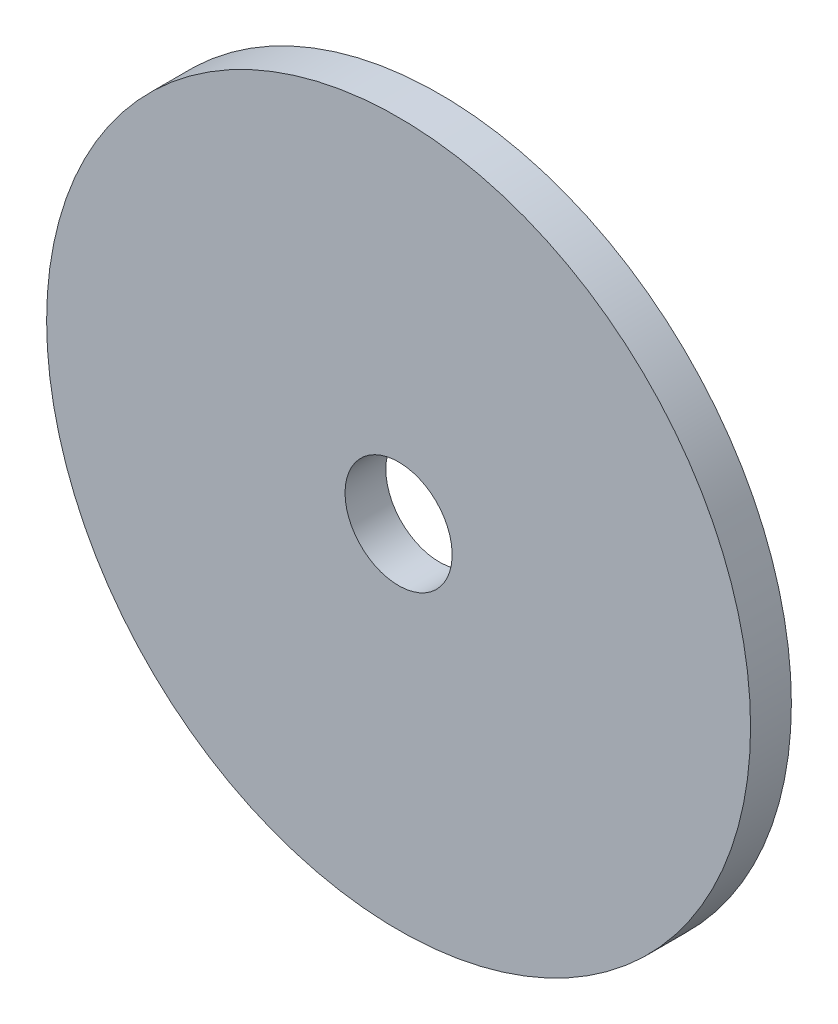
from build123d import *

# Parameters (mm, degrees)
SKETCH1_R               = 345
BOSS_EXTRUDE1_DEPTH     = 40
CUT_EXTRUDE3_DEPTH      = 490.540600972
CUT_EXTRUDE3_DEPTH_BACK = 490.540600972
SKETCH8_R               = 52.5


with BuildPart() as part:
    # Sketch1 → Boss-Extrude1 (new body)
    with BuildSketch(Plane.XY):
        Circle(SKETCH1_R)
    extrude(amount=BOSS_EXTRUDE1_DEPTH)

    # Sketch8 → Cut-Extrude3 (cut, two sides: drawn at the far end of the back side and taken through both)
    with BuildSketch(Plane(origin=(0, 0, 40), x_dir=(-1, 0, 0), z_dir=(0, 0, -1)).offset(-CUT_EXTRUDE3_DEPTH_BACK)):
        Circle(SKETCH8_R)
    extrude(amount=CUT_EXTRUDE3_DEPTH + CUT_EXTRUDE3_DEPTH_BACK, mode=Mode.SUBTRACT)


solid = part.part
